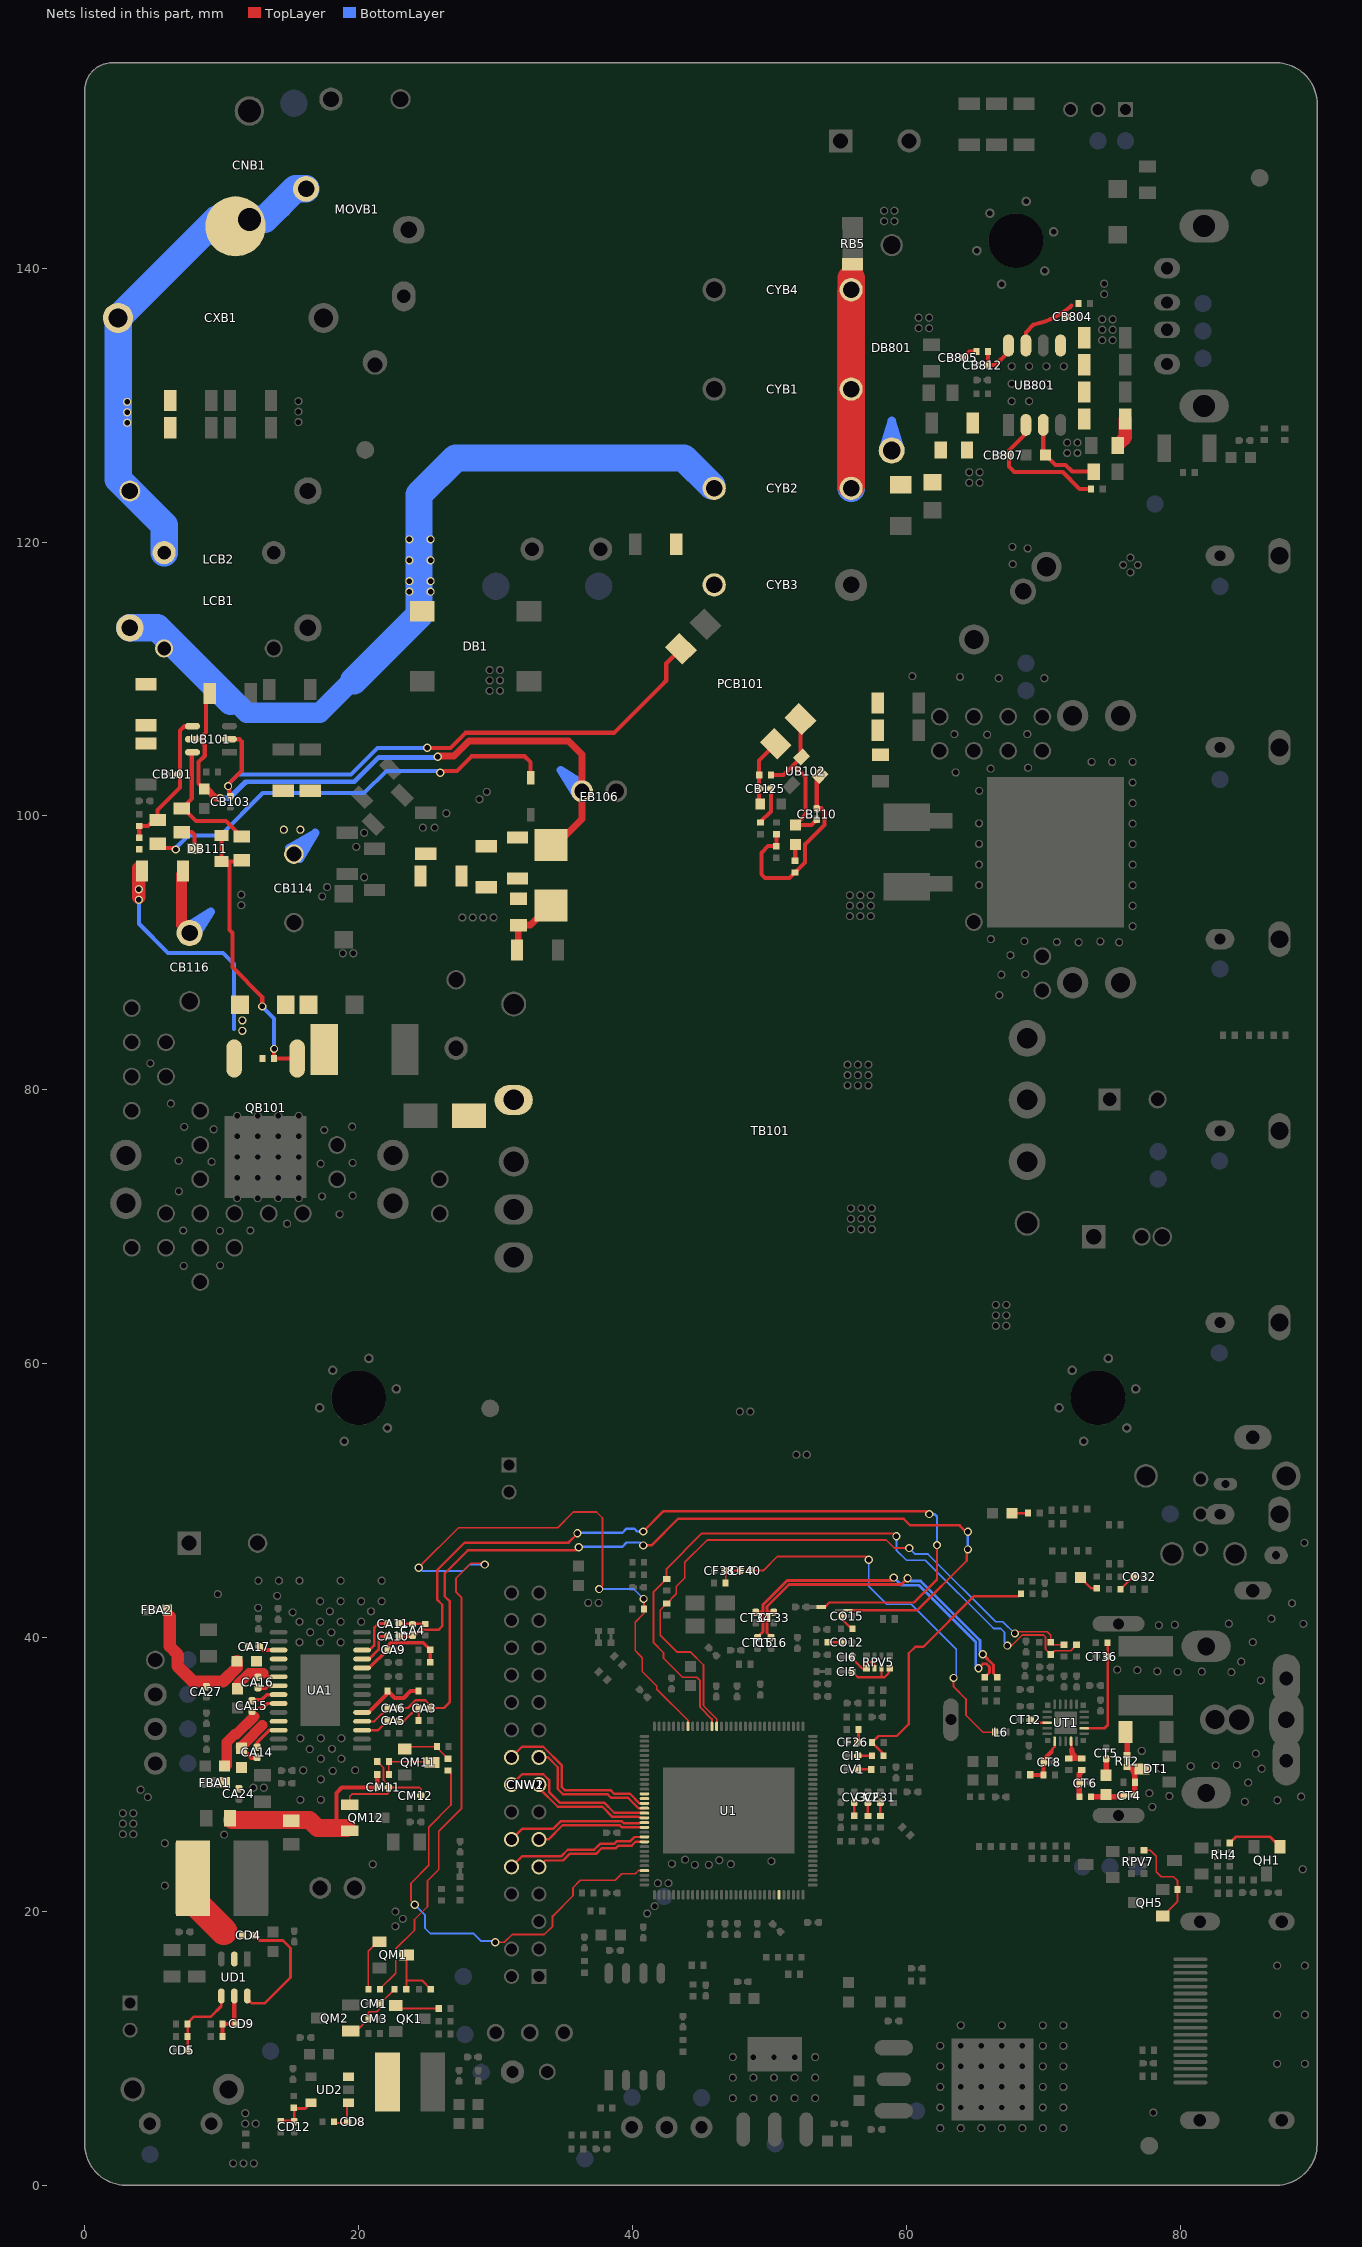
[diagram p0: the nets of this part, all layers, seen from the top]
# Altium PCB MISC116569.PcbDoc (part 11 of 15)
Units mm, origin at the board's own origin, x right, y up, seen from the top; angles counter-clockwise.
Board outline 90 x 155 mm, 2 copper layers (TopLayer, BottomLayer), stack 1.571 mm thick; 527 components, 277 nets, 2450 pads, 649 vias.

## Via types
v1: diameter 0.6, hole 0.4, TopLayer to BottomLayer, tented both sides, 649 vias

## Nets (pads, with @x,y where several pads share a name; then routed paths per layer and width w, separated by ;. In a path a pad name is that pad's centre, name@x,y a point inside that pad or via, vN(x,y) a via of type N, cw(c..) or ccw(c..) an arc to the next point about the centre after c; other vN are vias at no path point) (continued)
LVDS_O1N_IC: CNW1.9 CNW2.9 U1.87 | length 8.5
  TopLayer w0.178: CNW2.9@33.164,23.251 33.625,23.713 34.914,23.713 35.397,24.196 37.327,24.196 37.754,24.623 38.791,24.623 38.969,24.801 39.946,24.801 40.228,25.082 U1.87@40.873,25.082
LVDS_O1P_IC: CNW1.10 CNW2.10 U1.86 | length 10.6
  TopLayer w0.178: CNW2.10@31.164,23.251 31.755,23.843 31.93,24.017 34.788,24.017 35.271,24.501 37.201,24.501 37.628,24.928 38.665,24.928 38.843,25.106 39.82,25.106 40.147,25.432 U1.86@40.873,25.432
LVDS_O2N_IC: CNW1.11 CNW2.11 U1.84 | length 8.2
  TopLayer w0.178: CNW2.11@33.164,25.251 33.858,25.251 34.896,26.29 39.077,26.29 39.234,26.132 U1.84@40.873,26.132
LVDS_O2P_IC: CNW1.12 CNW2.12 U1.83 | length 10.3
  TopLayer w0.178: CNW2.12@31.164,25.251 31.93,26.017 34.193,26.017 34.77,26.595 39.203,26.595 39.361,26.437 40.477,26.437 40.522,26.482 U1.83@40.873,26.482
LVDS_O3N_IC: CNW1.17 CNW2.17 U1.80 | length 10.2
  TopLayer w0.178: CNW2.17@33.164,31.197 CNW2.17@33.164,31.251 33.816,31.251 34.539,30.528 34.539,29.821 34.539,28.934 34.921,28.552 38.182,28.552 38.448,28.285 39.688,28.285 40.441,27.532 U1.80@40.873,27.532
LVDS_O3P_IC: CNW1.18 CNW2.18 U1.79 | length 12.7
  TopLayer w0.178: CNW2.18@31.164,31.251 31.93,32.017 33.481,32.017 34.844,30.654 34.844,29.06 35.047,28.857 38.389,28.857 38.655,28.59 39.814,28.59 40.522,27.882 U1.79@40.873,27.882
LVDS_O4N_IC: U1.78
LVDS_O4P_IC: U1.77
LVDS_OCKN_IC: CNW1.15 CNW2.15 U1.82 | length 8.8
  TopLayer w0.178: CNW2.15@33.164,29.251 33.164,29.016 34.542,27.638 37.803,27.638 38.541,26.899 40.454,26.899 40.521,26.832 U1.82@40.873,26.832
LVDS_OCKP_IC: CNW1.16 CNW2.16 U1.81 | length 11.7
  TopLayer w0.178: CNW2.16@31.164,29.251 31.93,30.017 33.481,30.017 33.93,29.569 33.93,28.681 34.668,27.942 37.929,27.942 38.668,27.204 39.401,27.204 39.481,27.204 40.851,27.204 U1.81@40.873,27.182
MAIN_SCL_OUT_IC: DI11.K RF43.2 RT15.2 U1.52 | length 51
  TopLayer w0.127: U1.52@45.8,33.507 45.8,34.039 44.934,34.905 44.934,36.854 44.691,37.097 43.65,37.097 42.261,38.486 42.261,38.892 41.542,39.611 41.542,43.333 DI11.K@42.489,44.281 42.489,45.029 45.062,47.602 v1@59.061,47.602 ; v1@67.412,39.442 v1(67.381,39.412) 67.703,39.412 68.479,40.187 70.01,40.187 70.159,40.038 70.159,39.14 RF43.2@70.549,38.75 70.829,39.03 71.992,39.03 RT15.2@72.436,39.473 RT15.2@72.338,39.473
  BottomLayer w0.127: v1(59.272,47.391) 59.272,46.374 60.013,45.634 61.391,45.634 66.371,40.653 66.898,40.653 67.17,40.38 v1@67.17,39.623
MAIN_SDA_IO_IC: DI10.K RF44.2 RT14.2 U1.51 | length 47.1
  TopLayer w0.127: U1.51@46.149,33.508 46.149,34.049 45.188,35.01 45.188,37.994 44.246,38.936 43.259,38.936 42.024,40.17 42.024,42.012 DI10.K@42.489,42.477 43.2,43.188 43.2,43.725 43.823,44.347 43.823,45.492 45.45,47.119 58.527,47.119 59.111,46.535 v1(60.206,46.535) ; v1(67.928,40.294) 67.928,40.344 67.856,40.416 70.289,40.416 70.549,40.156 RF44.2@70.549,39.652 70.728,39.473 RT14.2@71.521,39.473
  BottomLayer w0.127: v1(60.206,46.535) 60.65,46.091 61.58,46.091 66.523,41.148 67.049,41.148 67.903,40.294 v1(67.928,40.294)
MHL_5V_IN_IC: U1.123
N-2: CNB1.3 CXB1.2 LCB1.2 LCB2.2 MOVB1.2@16.159,145.797 pad.VIA5@3.094,128.714 pad.VIA5@3.094,129.476 pad.VIA5@3.094,130.238 RB3.2 RB4.2 TP_N.1 | length 36.2
  BottomLayer w2: LCB1.2@5.793,119.231 5.793,121.231 LCB2.2@3.293,123.731 2.431,124.593 CXB1.2@2.431,136.373 8.287,142.228 9.623,143.564 CNB1.3@12.023,143.564 13.154,143.564 15.387,145.797 MOVB1.2@16.159,145.797
N-3: CYB2.1 DB1.3 LCB1.3 LCB2.3 pad.VIA5@23.706,116.383 pad.VIA5@23.706,117.145 pad.VIA5@23.706,118.669 pad.VIA5@23.706,120.193 pad.VIA5@25.251,116.383 pad.VIA5@25.251,117.145 pad.VIA5@25.251,118.669 pad.VIA5@25.251,120.193 RB141.2 | length 63.6
  BottomLayer w1.5: 8.12,111.257 11.846,107.531 17.164,107.531 ; 17.933,108.3 17.164,107.531 ; 19.65,109.876 19.508,109.876 17.164,107.531
  BottomLayer w2: LCB2.3@3.293,113.731 5.292,113.731 10.662,108.362 ; 19.65,109.876 24.406,114.632 24.406,117.145 24.406,120.193 24.406,123.448 27.098,126.14 43.747,126.14 CYB2.1@45.783,124.104
NetBA1_1: BA1.1 CA14.2@12.586,31.194 CA14.2@12.586,31.369 UA1.25 | length 3.7
  TopLayer w0.3: BA1.1@11.443,31.91 12.159,31.194 CA14.2@12.586,31.194
  TopLayer w0.762: BA1.1@11.402,32.019 11.704,32.322 ; 11.704,32.322 12.974,33.592
NetBA1_2: BA1.2 CA24.2@11.252,28.831 CA24.2@11.252,29.006 FBA1.1
NetBA2_1: BA2.1 CA15.2@12.205,34.572 CA15.2@12.205,34.747 UA1.23 | length 6
  TopLayer w0.254: 12.746,34.849 12.98,34.849 13.31,35.179 UA1.23@14.154,35.179
  TopLayer w0.762: BA2.1@10.38,30.664 10.38,32.337 10.967,32.924 11.073,32.924 12.379,34.23
NetBA3_1: BA3.1 CA16.2@12.649,36.972 CA16.2@12.649,37.148 UA1.20 | length 3
  TopLayer w0.254: 13.375,37.129 UA1.20@14.154,37.129
  TopLayer w0.762: BA3.1@11.151,36.534 11.999,37.382 13.03,37.382
NetBA4_1: BA4.1 CA17.2@11.936,39.332 CA17.2@12.111,39.332 UA1.18
NetBA4_2: BA4.2 CA27.1 FBA2.1 | length 9.5
  TopLayer w0.889: 6.201,41.529 6.201,39.355 6.776,38.78 6.776,37.915 7.899,36.792 10.097,36.792 11.125,37.82 BA4.2@11.125,38.265
NetBB101_2: BB101.2 TB101.3
NetBB801_2: BB801.2 BB802.2 CB810.1 DB801.A
NetCA3_1: CA3.1 CA6.1 RA4.JP_1K | length 65.8
  TopLayer w0.178: CA6.1@22.964,34.849 23.592,34.849 24.163,35.42 24.862,35.42 CA3.1@25.331,34.951 ; CA3.1@25.229,34.849 26.221,34.849 26.669,35.297 26.669,42.625 26.289,43.005 26.289,44.682 27.977,46.37 35.86,46.37 ; v1(40.787,46.726) 41.379,46.726 43.322,48.669 59.802,48.669 60.284,48.186 63.889,48.186 64.359,47.716 v1(64.498,47.716) ; RA4.JP_1K@55.969,41.997 60.803,41.997 64.409,45.604 64.409,46.345 v1(64.498,46.434)
  BottomLayer w0.178: v1@36.116,46.626 39.258,46.626 39.568,46.937 v1@40.576,46.937 ; v1(64.498,46.434) v1(64.498,47.716)
  other v1: 36.076,46.586
NetCA3_2: CA3.2@24.379,34.849 CA3.2@24.554,34.849 CA5.1 RA3.2 | length 2.7
  TopLayer w0.178: CA5.1@22.964,33.929 23.332,33.929 24.252,34.849 CA3.2@24.379,34.849 RA3.2@24.379,33.929
NetCA4_1: CA4.1 CA11.1 RA14.2 | length 1.9
  TopLayer w0.178: CA11.1@22.964,41.018 22.988,40.995 RA14.2@24.862,40.995
NetCA4_2: CA4.2@23.935,40.113 CA4.2@23.935,40.288 CA10.1 RA5.JP_1K | length 60
  TopLayer w0.178: CA10.1@22.964,40.063 23.884,40.063 CA4.2@23.935,40.113 24.086,40.113 24.533,40.56 ; 24.722,40.56 24.533,40.56 ; v1@35.974,47.573 35.33,46.929 27.745,46.929 25.73,44.914 25.73,42.773 26.11,42.394 26.11,40.831 25.839,40.56 24.533,40.56 ; v1(40.787,47.742) 42.273,49.228 61.45,49.228 ; RA5.JP_1K@53.785,42.23 54.046,42.23 54.373,42.556 60.571,42.556 62.238,44.223 v1(62.238,46.751)
  BottomLayer w0.178: v1@36.007,47.648 39.264,47.648 39.568,47.953 40.129,47.953 40.341,47.742 v1(40.787,47.742) ; v1(61.666,49.012) 62.06,49.012 62.238,48.834 v1(62.238,46.751)
  other v1: 35.974,47.615
NetCA5_2: CA5.2@22.114,33.929 CA5.2@22.289,33.929 UA1.3 | length 2.2
  TopLayer w0.152: UA1.3@20.204,33.229 UA1.3@20.254,33.229 21.415,33.229 CA5.2@22.114,33.929
NetCA6_2: CA6.2@22.114,34.849 CA6.2@22.289,34.849 UA1.4 | length 2.3
  TopLayer w0.152: UA1.4@20.254,33.879 21.144,33.879 CA6.2@22.114,34.849
NetCA9_2: CA9.2@22.114,39.107 CA9.2@22.289,39.107 RA10.2 RA11.2 UA1.10 | length 7
  TopLayer w0.254: UA1.10@20.254,37.779 20.786,37.779 CA9.2@22.114,39.107 22.114,39.401 22.335,39.622 22.71,39.622 24.714,39.622 RA11.2@25.229,39.107 RA10.2@25.229,38.195
NetCA10_2: CA10.2@22.114,40.101 CA10.2@22.289,40.101 UA1.11 | length 3
  TopLayer w0.203: UA1.11@20.254,38.429 20.771,38.429 21.463,39.121 21.463,39.895 21.63,40.063 CA10.2@22.114,40.063
NetCA11_2: CA11.2@22.114,41.018 CA11.2@22.289,41.018 UA1.12 | length 3.5
  TopLayer w0.203: UA1.12@20.204,39.079 20.799,39.079 21.132,39.413 21.132,40.695 21.455,41.018 CA11.2@22.114,41.018
NetCA14_1: CA14.1 UA1.26 | length 2.3
  TopLayer w0.254: CA14.1@12.586,32.044 12.586,32.342 13.473,33.229 UA1.26@14.154,33.229 ; CA14.1@12.716,31.991 CA14.1@12.716,32.044
NetCA15_1: CA15.1 UA1.22 | length 2.1
  TopLayer w0.254: CA15.1@12.243,35.439 12.896,35.439 13.287,35.829 UA1.22@14.154,35.829
NetCA16_1: CA16.1 UA1.21 | length 1.6
  TopLayer w0.254: CA16.1@12.649,36.298 13.217,36.298 13.398,36.479 UA1.21@14.154,36.479
NetCA17_1: CA17.1 UA1.17 | length 1.5
  TopLayer w0.305: CA17.1@12.786,39.332 13.039,39.079 UA1.17@14.154,39.079
NetCA31_1: CA31.1 RA33.1 | length 1.2
  TopLayer w0.178: CA31.1@67.707,49.075 67.719,49.088 RA33.1@68.893,49.088
NetCA32_1: CA32.1 RA34.1 | length 1.5
  TopLayer w0.178: CA32.1@72.707,44.375 73.483,43.6 RA34.1@73.901,43.6
NetCB101_1: CB101.1 RB103.2 RB105.1 RB121.2 UB101.4 | length 10.5
  TopLayer w0.3: RB105.1@3.975,98.412 RB103.2@3.975,99.27 4.604,99.27 RB121.2@5.194,99.86 ; RB121.2@5.309,99.746 5.309,100.443 6.954,102.089 6.954,103.683 6.954,106.23 7.275,106.55 UB101.4@7.858,106.55
NetCB102_1: CB102.1 DB104.K EB106.1 RB102.2 RB116.1 RB163.2 UB101.5 | length 45.7
  TopLayer w0.3: UB101.5@7.858,105.6 8.357,105.6 8.865,106.109 RB102.2@8.865,109.24 ; UB101.5@8.344,105.6 8.761,105.184 8.761,104.379 8.317,103.936 8.317,102.358 CB102.1@8.725,101.951 CB102.1@8.761,101.987
  TopLayer w0.5: CB102.1@8.725,101.951 8.92,101.951 9.563,101.308 v1(9.893,101.308) ; v1@25.781,104.37 26.958,104.37 28.057,105.469 35.323,105.469 36.311,104.481 EB106.1@36.311,101.803 EB106.1@36.311,101.486 ; DB104.K@34.965,98.426 36.311,99.773 EB106.1@36.311,101.486 ; EB106.1@36.47,101.644 EB106.1@36.311,101.486
  BottomLayer w0.35: 11.744,102.469 11.775,102.5 19.691,102.5 ; 19.937,102.745 19.691,102.5 ; v1@25.733,104.27 21.461,104.27 19.691,102.5
  BottomLayer w0.4: v1(9.893,101.308) 10.583,101.308 11.744,102.469 ; v1@25.733,104.27 v1(25.781,104.318)
NetCB103_2: CB103.2@10.63,101.291 CB103.2@10.63,101.466 PCB101.4 UB101.2 | length 43.5
  TopLayer w0.3: UB101.2@10.558,105.6 11.29,105.6 11.461,105.43 11.461,103.293 10.465,102.298 v1(10.465,102.184) 10.546,102.103 10.546,101.55 CB103.2@10.63,101.466 ; v1(25.008,104.973) 25.204,104.973 26.708,104.973 27.807,106.072 38.66,106.072 42.151,109.563 42.464,109.876 42.464,111.133 PCB101.4@43.537,112.206
  BottomLayer w0.3: v1(10.465,102.184) 10.465,102.298 11.195,103.028 19.437,103.028 21.382,104.973 v1(25.008,104.973) v1@24.977,105.004
NetCB109_1: CB109.1 CB110.1 PCB101.2 RB132.1 UB102.K | length 13
  TopLayer w0.3: RB132.1@50.102,102.984 51.024,102.984 51.751,103.711 ; UB102.K@52.262,104.387 PCB101.2@52.262,107.072 52.357,106.977 52.357,106.693 PCB101.2@52.633,106.417 ; UB102.K@52.345,104.305 51.751,103.711 ; CB110.1@53.454,99.708 53.086,99.339 CB109.1@51.887,99.339 52.633,100.085 52.633,102.83 51.751,103.711
NetCB109_2: CB109.2 RB133.1 | length 1.2
  TopLayer w0.3: RB133.1@51.887,96.749 CB109.2@51.887,97.927
NetCB110_2: CB110.2@53.454,100.383 CB110.2@53.454,100.558 RB133.2 RB134.2 RB135.2 UB102.R | length 15.3
  TopLayer w0.3: 49.424,96.716 49.424,97.028 ; RB135.2@50.516,98.667 50.503,98.655 RB134.2@50.503,97.79 49.906,97.79 49.424,97.307 49.424,97.028 ; UB102.R@53.692,102.958 53.454,102.721 CB110.2@53.454,100.558 53.785,100.558 54.013,100.33 54.013,99.339 52.603,97.93 52.603,96.598 51.879,95.873 RB133.2@51.862,95.873 51.467,95.479 49.682,95.479 49.424,95.737 49.424,97.028
NetCB113_1: CB113.1 DB104.A RB114.1 | length 4.7
  TopLayer w0.5: RB114.1@31.559,90.208 31.661,90.31 CB113.1@31.661,92.023 32.537,92.023 DB104.A@33.961,93.448
NetCB113_2: CB113.2 RB116.2
NetCB114_1: CB114.1@15.269,97.209 pad.VIA5@14.541,98.996 pad.VIA5@15.748,98.996 RB117.1 RB118.1
NetCB116_1: CB116.1 RB119.2 | length 4.5
  TopLayer w0.8: RB119.2@7.061,95.707 7.061,92.047 CB116.1@7.658,91.451
NetCB118_2: CB118.2 RB123.1 RB124.1
NetCB125_1: CB125.1 PCB101.1 RB131.1 RB132.2 | length 5
  TopLayer w0.3: RB131.1@49.34,100.863 49.252,100.951 CB125.1@49.253,101.994 RB132.2@49.252,102.984 49.252,104.062 PCB101.1@50.466,105.276
NetCB125_2: CB125.2@49.927,101.994 CB125.2@50.103,101.994 RB158.1 | length 2.8
  TopLayer w0.3: RB158.1@49.347,99.517 49.347,99.581 50.103,100.336 CB125.2@50.103,101.994
NetCB801_1: CB801.1 RB816.2 UB801.3 | length 8
  TopLayer w0.3: 69.997,126.845 UB801.3@69.997,128.558 69.997,126.528 CB801.1@70.163,126.362 70.894,125.631 71.63,125.631 72.115,125.146 RB816.2@73.691,125.146
NetCB804_2: CB804.2@71.673,136.449 CB804.2@71.848,136.449 RB805.1 UB801.7 | length 5
  TopLayer w0.3: UB801.7@68.728,134.358 68.728,135.319 69.296,135.887 69.308,135.887 ; 69.324,135.89 ccw(c68,142.004) 71.932,137.138 ; 71.915,137.122 71.932,137.138 ; 72.073,137.28 71.932,137.138 ; 69.309,135.887 ccw(c68,142.004) 69.323,135.89 69.312,135.89 69.308,135.887
NetCB805_1: CB805.1 RB804.2 | length 1.1
  TopLayer w0.3: CB805.1@64.17,133.477 64.615,133.921 RB804.2@65.115,133.921
NetCB807_2: CB807.2@67.327,126.34 CB807.2@67.501,126.34 RB801.2 UB801.2 | length 11.3
  TopLayer w0.3: 67.819,127.015 68.564,127.76 ; UB801.2@68.728,128.558 68.728,127.924 68.564,127.76 ; RB801.2@73.49,123.888 72.661,123.888 71.422,125.127 67.882,125.127 67.501,125.508 CB807.2@67.501,126.34 67.501,126.698 68.564,127.76
NetCB809_1: CB809.1 RB810.2 | length 2
  TopLayer w1: CB809.1@75.522,127.177 75.993,127.648 RB810.2@75.993,128.981
NetCB810_2: CB810.2 RB812.1
NetCB812_1: CB812.1 RB804.1 UB801.8 | length 3.4
  TopLayer w0.3: RB804.1@65.965,133.921 CB812.1@65.965,132.918 66.492,132.918 67.457,133.883 UB801.8@67.457,134.358
NetCD4_1: CD4.1 LD1.1 LD3.2 UD1.2 | length 4.9
  TopLayer w2: LD3.2@7.657,22.424 7.657,21.033 10.158,18.532
NetCD4_2: CD4.2@12.171,18.25 CD4.2@12.346,18.25 UD1.6 | length 9.4
  TopLayer w0.203: UD1.6@11.867,13.825 11.867,13.642 12.225,13.284 13.134,13.284 15.019,15.169 15.019,17.31 14.463,17.866 12.768,17.866 CD4.2@12.422,18.212
NetCD5_1: CD5.1 RD3.1 RD5.2 UD1.4 | length 5.7
  TopLayer w0.203: CD5.1@7.513,9.868 7.513,11.836 7.985,12.308 9.204,12.308 9.967,13.071 UD1.4@9.967,13.825
NetCD8_2: CD8.2@19.149,4.638 CD8.2@19.324,4.638 RD7.1 UD2.1 | length 2.3
  TopLayer w0.127: RD7.1@18.207,4.549 19.149,4.549 UD2.1@19.149,5.9
NetCD9_2: CD9.2@11.009,11.786 CD9.2@11.184,11.786 RD1.2 RD6.2 UD1.5 | length 4
  TopLayer w0.305: RD1.2@10.054,10.858 RD6.2@10.054,11.773 10.996,11.773 CD9.2@11.009,11.786 10.917,11.877 UD1.5@10.917,13.825
NetCD12_1: CD12.1 RD8.1 RD9.2 UD2.5 | length 3.3
  TopLayer w0.203: RD9.2@14.308,4.695 CD12.1@15.299,4.695 15.299,4.8 RD8.1@15.299,5.569 ; RD8.1@15.261,5.608 16.106,5.608 UD2.5@16.524,6.025
NetCF26_2: CF26.2@56.32,32.36 CF26.2@56.496,32.36 RF12.1 | length 0.9
  TopLayer w0.203: CF26.2@56.496,32.36 RF12.1@56.496,33.287
NetCF31_2: CF31.2@58.102,27.909 CF31.2@58.102,28.084 RF16.1 | length 0.9
  TopLayer w0.178: RF16.1@58.102,26.962 CF31.2@58.102,27.909
NetCF38_2: CF38.2@46.626,44.884 CF38.2@46.801,44.884 CF40.2@47.849,44.884 CF40.2@48.024,44.884 RF25.1 | length 2
  TopLayer w0.127: RF25.1@46.8,43.97 CF38.2@46.801,44.884 CF40.2@47.849,44.884
NetCF40_1: CF40.1 L6.1 | length 27.6
  TopLayer w0.127: CF40.1@48.699,44.884 49.546,44.884 50.575,45.913 53.805,45.913 ; 54.148,45.913 53.805,45.913 ; v1(57.247,45.672) 57.247,45.722 57.056,45.913 53.805,45.913 ; v1(63.449,37.046) 63.449,36.412 64.359,35.502 64.359,34.328 65.601,33.086 L6.1@66.474,33.086
  BottomLayer w0.127: v1(57.247,45.672) 57.247,43.741 58.555,42.433 60.345,42.433 63.643,39.136 63.643,37.239 v1(63.449,37.046)
NetCI1_2: CI1.2@56.312,31.355 CI1.2@56.487,31.355 RI3.2 | length 1.2
  TopLayer w0.178: CI1.2@56.326,31.369 RI3.2@57.487,31.369
NetCI5_2: CI5.2@55.896,37.506 CI5.2@56.071,37.506 RPV5.5 RPV5.7 | length 4
  TopLayer w0.178: CI5.2@56.04,37.506 56.449,37.097 58.395,37.097 58.712,37.414 58.712,37.674 RPV5.7@58.786,37.749 ; 58.186,37.114 RPV5.5@58.186,37.749
NetCI6_2: CI6.2@55.896,38.572 CI6.2@56.071,38.572 RPV5.1 RPV5.3 | length 2.8
  TopLayer w0.127: RPV5.1@57.086,37.749 57.086,38.095 57.196,38.204 57.602,38.204 57.686,38.12 RPV5.3@57.686,37.749
  TopLayer w0.178: CI6.2@56.071,38.572 56.071,38.452 56.775,37.749 RPV5.1@57.086,37.749
NetCM1_1: CM1.1 CM3.2@20.709,12.141 CM3.2@20.884,12.141 QM2.G RM4.2 | length 5.5
  TopLayer w0.127: QM2.G@18.848,11.255 19.823,11.255 CM3.2@20.709,12.141 20.709,12.599 20.785,12.675 21.331,12.675 21.559,12.903 CM1.1@21.559,13.266 21.583,13.266 RM4.2@22.63,14.313
NetCM11_1: CM11.1 CM12.2@24.4,28.448 CM12.2@24.576,28.448 QM12.G RM14.2 | length 9.1
  TopLayer w0.127: QM12.G@19.356,27.785 19.356,28.404 19.515,28.562 22.08,28.562 22.207,28.689 CM11.1@22.207,29.046 ; RM14.2@21.357,30.932 21.814,30.476 21.814,29.591 22.207,29.197 CM11.1@22.207,29.046 ; CM12.2@24.576,28.448 24.576,28.912 24.441,29.046 CM11.1@22.207,29.046
NetCM11_2: CM11.2@21.357,29.046 CM11.2@21.532,29.046 QM12.S R5V.2 R12V.2 RM13.1 | length 15.3
  TopLayer w0.305: 18.372,26.126 18.372,28.651 18.767,29.046 CM11.2@21.357,29.046 RM13.1@21.357,29.989
  TopLayer w1.321: R12V.2@10.742,26.673 16.401,26.673 16.988,26.086 QM12.S@19.156,26.086
NetCO12_1: CO12.1 RO12.2 | length 1
  TopLayer w0.178: RO12.2@54.205,39.652 CO12.1@55.221,39.652
NetCO15_1: CO15.1 RO15.2 | length 1.3
  TopLayer w0.178: CO15.1@55.222,41.557 55.222,41.41 55.989,40.642 RO15.2@56.071,40.642
NetCO32_1: CO32.1 RI16.1 | length 1.3
  TopLayer w0.178: RI16.1@75.642,43.523 75.645,43.523 CO32.1@76.574,44.452
NetCT3_1: CT3.1 RT2.1 | length 1.5
  TopLayer w0.401: CT3.1@76.003,32.921 76.132,32.792 RT2.1@76.132,31.49
NetCT4_1: CT4.1 CT7.2 LT2.1 | length 2.3
  TopLayer w0.401: CT7.2@73.49,28.374 CT4.1@75.77,28.374
NetCT4_2: CT4.2@76.521,28.45 CT4.2@76.696,28.45 DT1.2 LT1.2 RT2.2 RT2.3 | length 2.4
  TopLayer w0.401: RT2.2@76.119,30.553 76.149,30.553 cw(c76.149,30.183) 76.411,30.444 cw(c75.722,29.755) 76.696,29.755 CT4.2@76.696,28.45
NetCT5_1: CT5.1 LT2.2 | length 1.1
  TopLayer w0.401: LT2.2@74.595,29.982 CT5.1@74.595,31.112
NetCT6_1: CT6.1 CT7.1 LT3.1 | length 2
  TopLayer w0.401: CT7.1@72.64,28.374 72.64,30.039 72.817,30.216 LT3.1@72.817,30.324
NetCT8_1: CT8.1 CT9.2 FT2.1 UT1.20 | length 3.8
  TopLayer w0.178: 70.642,31.625 70.642,31.834 70.832,32.024 UT1.20@70.832,32.422
  TopLayer w0.305: FT2.1@69.045,29.962 70.014,29.962 CT9.2@70.016,29.96 ; CT9.2@70.024,29.96 70.024,31.097 70.578,31.651
NetCT12_2: CT12.2@68.933,33.988 CT12.2@69.108,33.988 UT1.16 | length 1.3
  TopLayer w0.178: CT12.2@69.108,33.988 69.324,33.772 UT1.16@70.282,33.772
NetCT15_1: CT15.1 CT34.1 RT10.2 | length 24.9
  TopLayer w0.203: CT34.1@49.002,41.881 49.493,41.881 ; CT15.1@49.136,40.03 49.525,40.419 49.525,42.389 51.305,44.169 v1@58.983,44.169 ; v1(65.268,37.76) 65.584,38.075 65.85,38.075 66.065,37.859 66.065,37.442 RT10.2@65.724,37.101 RT10.2@65.724,37.146
  BottomLayer w0.203: v1(59.075,44.376) 59.634,43.817 60.919,43.817 65.07,39.666 v1@65.07,37.864
NetCT16_2: CT16.2@50.127,39.855 CT16.2@50.127,40.03 CT33.2@50.31,41.706 CT33.2@50.31,41.881 RT13.2 | length 24.4
  TopLayer w0.203: CT16.2@50.127,40.03 49.83,40.327 49.83,41.925 ; CT33.2@50.31,41.881 49.874,41.881 49.83,41.925 ; v1(60.091,44.325) 59.63,43.864 51.432,43.864 49.83,42.263 49.83,41.925 ; v1(65.583,38.773) 66.37,37.986 66.37,37.369 RT13.2@66.638,37.101
  BottomLayer w0.203: v1@60.091,44.224 v1(60.091,44.325) 60.295,44.122 61.045,44.122 65.375,39.792 65.375,38.981 v1(65.583,38.773)
NetCT36_1: CT36.1 RT5.2 UT1.3 | length 8.3
  TopLayer w0.178: UT1.3@72.982,33.372 73.558,33.372 74.056,33.372
  TopLayer w0.203: 73.558,33.372 74.482,33.372 74.709,33.599 RT5.2@74.709,39.584
NetCV1_1: CV1.1 RV2.2 | length 0.9
  TopLayer w0.178: CV1.1@56.487,30.366 RV2.2@57.434,30.366
NetCV2_1: CV2.1 RV4.2 | length 1.1
  TopLayer w0.178: RV4.2@57.188,26.962 CV2.1@57.188,28.084
NetCV3_1: CV3.1 RV10.2 | length 0.9
  TopLayer w0.178: RV10.2@56.195,26.983 56.197,26.985 CV3.1@56.197,27.909
NetCYB1_2: CYB1.2 CYB2.2 CYB4.2 RB5.1 | length 29.5
  TopLayer w2: CYB2.2@55.964,124.117 CYB4.2@55.964,139.268
  BottomLayer w2: CYB2.2@55.964,123.924 CYB4.2@55.964,138.239
NetCYB3_1: CYB3.1 RB130.2
NetDB109_A: DB109.A pad.VIA5@3.95,93.878 pad.VIA5@3.95,94.64 pad.VIA5@11.506,84.303 pad.VIA5@11.506,85.065 QB101.S RB105.2 RB109.2 RB119.1 RB148.2 | length 17.6
  TopLayer w1: pad.VIA5@3.95,94.056 RB119.1@3.95,96.19
  BottomLayer w0.3: pad.VIA5@3.95,94.64 pad.VIA5@3.95,93.878 3.95,92.126 6.078,89.998 10.091,89.998 10.907,89.182 10.907,84.427
NetDB109_K: DB109.K DB110.A
NetDB111_1: DB111.1 DB111.3 QB101.G RB106.2 RB109.1 | length 20.8
  TopLayer w0.3: DB111.3@9.982,98.59 9.982,96.685 10.579,96.685 ; RB106.2@11.455,96.772 11.369,96.685 10.579,96.685 ; v1(12.956,86.084) 12.956,86.789 10.795,88.951 10.795,91.465 10.579,91.681 10.579,96.685 ; v1(13.824,82.989) RB109.1@13.824,82.283 QB101.G@15.507,82.283
  BottomLayer w0.3: v1(12.956,86.084) 13.824,85.217 v1(13.824,82.989)
NetDB111_2: DB111.2 RB107.2 | length 2.1
  TopLayer w0.3: RB107.2@6.985,98.816 7.813,98.816 8,98.629 DB111.2@8,97.612
NetDB121_K: DB121.K RB121.1 | length 32.6
  TopLayer w0.3: RB121.1@5.443,98.014 5.309,98.014 5.418,97.904 5.672,97.65 v1@6.642,97.65 ; v1(25.954,103.149) 26.094,103.289 27.178,103.289 28.245,104.356 32.131,104.356 32.563,103.924 DB121.K@32.563,102.789
  BottomLayer w0.3: v1@6.642,97.65 7.569,98.577 9.906,98.577 12.995,101.667 20.405,101.667 22.027,103.289 24.066,103.289 ; 24.879,103.289 24.066,103.289 ; v1(25.954,103.149) 25.814,103.289 24.066,103.289
  other v1: 6.642,97.549
NetLD2_2: LD2.2 UD2.3
NetLT3_2: LT3.2 LT4.2 UT1.23 | length 2.3
  TopLayer w0.178: 72.017,31.816 ccw(c71.981,31.852) 72.032,31.852 UT1.23@72.032,32.422
  TopLayer w0.401: LT4.2@71.852,31.174 72.423,31.174 ; 72.068,31.803 ccw(c72.728,31.803) 72.261,31.336 72.423,31.174 ; LT3.2@72.817,31.174 72.423,31.174
NetQH1_B: QH1.B RH4.7 | length 4.1
  TopLayer w0.203: RH4.7@83.622,24.994 84.073,25.445 86.554,25.445 QH1.B@87.282,24.717
NetQH5_B: QH5.B RH59.2 RPV7.2 | length 7.1
  TopLayer w0.127: RPV7.2@77.351,24.458 77.818,24.458 78.252,24.023 78.252,22.888 78.608,22.532 79.51,22.532 79.809,22.233 RH59.2@79.809,21.605 79.809,20.736 78.748,19.675 QH5.B@78.735,19.675
NetQK1_B: QK1.B RK15.1 | length 3.1
  TopLayer w0.127: QK1.B@22.753,12.906 RK15.1@25.853,12.906
NetQM1_B: QM1.B RM2.2 | length 4
  TopLayer w0.127: RM2.2@20.71,14.313 20.71,17.082 21.407,17.78 QM1.B@21.522,17.78 QM1.B@21.464,17.723
NetQM1_C: QM1.C RM3.1 RM4.1 | length 4.5
  TopLayer w0.152: QM1.C@23.504,16.815 23.504,14.948 ; RM4.1@23.505,14.313 23.504,14.315 23.504,14.948 ; RM3.1@25.267,14.313 24.633,14.948 23.504,14.948
NetQM11_B: QM11.B RM11.2 RM12.1 | length 3.4
  TopLayer w0.127: QM11.B@23.528,32.029 RM12.1@25.719,32.029 25.719,31.952 RM11.2@26.525,31.146
NetQM11_C: QM11.C RM13.2 RM14.1 | length 4
  TopLayer w0.127: RM13.2@22.207,29.989 RM14.1@22.207,30.932 QM11.C@25.299,30.932
NetRA8_2: RA8.2 RA9.2 UA1.5 | length 5.3
  TopLayer w0.305: UA1.5@20.254,34.529 20.732,34.529 22.114,35.911 RA8.2@22.114,36.087 22.13,36.087 22.634,35.583 23.294,35.583 23.798,36.087 RA9.2@24.379,36.087
NetRB106_1: RB106.1 RB107.1 UB101.6 | length 9.2
  TopLayer w0.3: RB107.1@6.985,100.548 7.102,100.548 7.814,101.261 7.814,104.607 UB101.6@7.858,104.65 ; RB107.1@7.506,100.266 8.133,99.639 10.32,99.639 RB106.1@11.455,98.504
NetRB141_1: RB141.1 RB142.2
NetRB161_2: RB161.2 RB162.1
NetRB162_2: RB162.2 RB163.1
NetRB810_1: RB810.1 RB818.2 RB819.2 RB820.2 UB801.5
NetRI3_1: RI3.1 RI15.2 RI18.2 | length 20.1
  TopLayer w0.178: RI3.1@58.337,31.493 RI18.2@57.496,32.334 57.966,32.804 59.302,32.804 60.178,33.68 60.178,38.845 60.655,39.321 61.252,39.321 64.95,43.019 65.46,43.019 ; 65.489,43.019 67.132,43.019 ; 66.598,43.019 67.132,43.019 ; 67.369,43.019 67.132,43.019 ; RI15.2@68.198,43.019 67.132,43.019
PANEL_EN_OUT_IC: RM11.1 U1.93 | length 32.7
  TopLayer w0.127: v1(24.1,20.485) 23.82,20.765 23.82,22.06 25.12,23.359 25.12,26.15 26.745,27.776 26.745,30.077 RM11.1@26.525,30.296 ; v1(29.98,17.744) 30.645,17.744 31.209,18.308 33.555,18.308 34.162,18.915 34.162,19.655 35.654,21.147 35.654,21.723 36.197,22.266 38.733,22.266 39.211,22.743 40.203,22.743 40.442,22.982 U1.93@40.873,22.982 U1.93@40.925,22.982
  BottomLayer w0.127: v1@24.061,20.447 v1(24.1,20.485) 24.839,19.746 24.839,18.786 25.25,18.375 28.412,18.375 28.959,17.828 29.896,17.828 v1(29.98,17.744)
POWER_EN_OUT_IC: RM1.1 RM2.1 U1.57 | length 75.4
  TopLayer w0.127: RM2.1@21.56,14.313 21.56,14.338 22.704,15.482 22.704,17.256 24.079,18.631 24.079,19.406 25.029,20.356 25.029,22.228 25.856,23.054 25.856,25.845 27.507,27.496 27.507,42.937 27.102,43.342 27.102,44.31 28.207,45.415 v1@29.11,45.415 ; v1(24.397,45.098) 24.397,45.125 27.293,48.021 34.537,48.021 35.686,49.17 37.367,49.17 37.808,48.729 37.808,43.784 v1(37.562,43.538) ; RM1.1@40.826,41.951 40.826,41.753 40.195,41.123 40.195,39.053 40.5,38.749 40.5,38.729 40.718,38.511 40.718,37.52 41.777,36.461 41.777,36.233 44.049,33.96 U1.57@44.049,33.508 U1.57@43.999,33.558 ; RM1.1@40.831,42.078 v1@40.831,42.796
  BottomLayer w0.127: v1(24.397,45.098) 24.64,44.854 27.646,44.854 28.119,45.327 v1@29.198,45.327 ; v1(37.562,43.538) 40.089,43.538 v1(40.813,42.814)
  other v1: 29.204,45.321